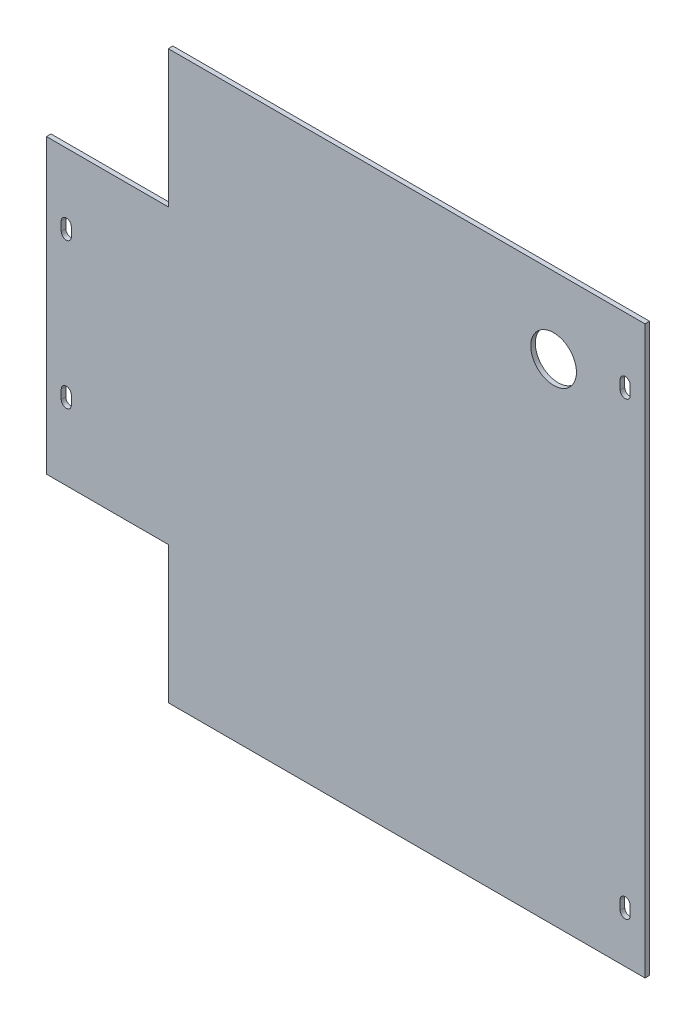
from build123d import *

# Parameters (mm, degrees)
SKETCH_1_W          = 363
SKETCH_1_H          = 372
EXTRUDE_1_DEPTH     = 3
SKETCH_2_R          = 15
CUT_EXTRUDE_1_DEPTH = 10
SKETCH_3_W          = 50
SKETCH_3_H          = 90
CUT_EXTRUDE_2_DEPTH = 10
SKETCH_4_W          = 3
SKETCH_4_H          = 192
EXTRUDE_2_DEPTH     = 30
CUT_EXTRUDE_3_DEPTH = 10


with BuildPart() as part:
    # 草图1 → 凸台-拉伸1 (new body)
    with BuildSketch(Plane.XY):
        Rectangle(SKETCH_1_W, SKETCH_1_H)
    extrude(amount=EXTRUDE_1_DEPTH)

    # 草图2 → 切除-拉伸1 (cut)
    with BuildSketch(Plane.XY.offset(3)):
        with Locations((121.5, 136)):
            Circle(SKETCH_2_R)
    extrude(amount=-CUT_EXTRUDE_1_DEPTH, mode=Mode.SUBTRACT)

    # 草图3 → 切除-拉伸2 (cut)
    with BuildSketch(Plane.XY.offset(3)):
        with Locations((-156.5, -141)):
            Rectangle(SKETCH_3_W, SKETCH_3_H)
        with Locations((-156.5, 141)):
            Rectangle(SKETCH_3_W, SKETCH_3_H)
    extrude(amount=-CUT_EXTRUDE_2_DEPTH, mode=Mode.SUBTRACT)

    # 草图4 → 凸台-拉伸2 (add)
    with BuildSketch(Plane.ZY.offset(181.5)):
        with Locations((1.5, 0)):
            Rectangle(SKETCH_4_W, SKETCH_4_H)
    extrude(amount=EXTRUDE_2_DEPTH)

    # 草图5 → 切除-拉伸3 (cut)
    with BuildSketch(Plane.XY.offset(3)):
        with BuildLine():
            Line((165.2, -155.557904139), (165.2, -149.557904139))
            ThreePointArc((165.2, -149.557904139), (168.5, -146.257904139), (171.8, -149.557904139))
            Line((171.8, -149.557904139), (171.8, -155.557904139))
            ThreePointArc((171.8, -155.557904139), (168.5, -158.857904139), (165.2, -155.557904139))
        make_face()
        with BuildLine():
            Line((165.2, 140.283744441), (165.2, 146.283744441))
            ThreePointArc((165.2, 146.283744441), (168.5, 149.583744441), (171.8, 146.283744441))
            Line((171.8, 146.283744441), (171.8, 140.283744441))
            ThreePointArc((171.8, 140.283744441), (168.5, 136.983744441), (165.2, 140.283744441))
        make_face()
        with BuildLine():
            Line((-195.2, 52.919675482), (-195.2, 46.919675482))
            ThreePointArc((-195.2, 46.919675482), (-198.5, 43.619675482), (-201.8, 46.919675482))
            Line((-201.8, 46.919675482), (-201.8, 52.919675482))
            ThreePointArc((-201.8, 52.919675482), (-198.5, 56.219675482), (-195.2, 52.919675482))
        make_face()
        with BuildLine():
            Line((-201.8, -48.714858664), (-201.8, -42.714858664))
            ThreePointArc((-201.8, -42.714858664), (-198.5, -39.414858664), (-195.2, -42.714858664))
            Line((-195.2, -42.714858664), (-195.2, -48.714858664))
            ThreePointArc((-195.2, -48.714858664), (-198.5, -52.014858664), (-201.8, -48.714858664))
        make_face()
    extrude(amount=-CUT_EXTRUDE_3_DEPTH, mode=Mode.SUBTRACT)


solid = part.part
